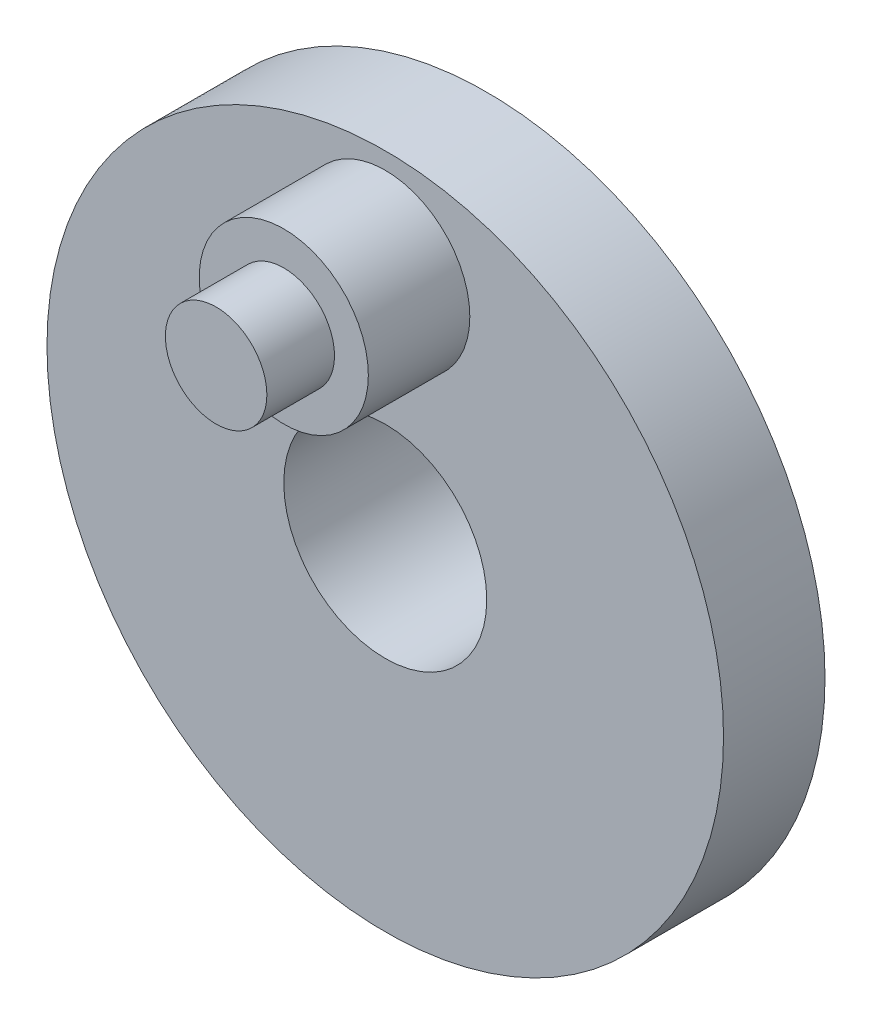
from build123d import *

# Parameters (mm, degrees)
SKETCH1_R           = 10
BOSS_EXTRUDE1_DEPTH = 3
SKETCH2_R           = 2.5
BOSS_EXTRUDE2_DEPTH = 3
SKETCH3_R           = 1.5
BOSS_EXTRUDE3_DEPTH = 2
SKETCH4_R           = 3
CUT_EXTRUDE1_DEPTH  = 24
BOSS_EXTRUDE4_START = 4
SKETCH5_R           = 4
SKETCH5_R_2         = 3
BOSS_EXTRUDE4_DEPTH = 4
SKETCH6_R           = 1
CUT_EXTRUDE2_DEPTH  = 5


with BuildPart() as part:
    # Sketch1 → Boss-Extrude1 (new body)
    with BuildSketch(Plane.XY):
        Circle(SKETCH1_R)
    extrude(amount=BOSS_EXTRUDE1_DEPTH)

    # Sketch2 → Boss-Extrude2 (add)
    with BuildSketch(Plane.XY.offset(3)):
        with Locations((0, 7)):
            Circle(SKETCH2_R)
    extrude(amount=BOSS_EXTRUDE2_DEPTH)

    # Sketch3 → Boss-Extrude3 (add)
    with BuildSketch(Plane.XY.offset(6)):
        with Locations((0, 7)):
            Circle(SKETCH3_R)
    extrude(amount=BOSS_EXTRUDE3_DEPTH)

    # Sketch4 → Cut-Extrude1 (cut)
    with BuildSketch(Plane(origin=(0, 0, 0), x_dir=(-1, 0, 0), z_dir=(0, 0, -1))):
        Circle(SKETCH4_R)
    extrude(amount=-CUT_EXTRUDE1_DEPTH, mode=Mode.SUBTRACT)

    # Sketch5 → Boss-Extrude4 (add)
    with BuildSketch(Plane(origin=(0, 0, 0), x_dir=(-1, 0, 0), z_dir=(0, 0, -1)).offset(BOSS_EXTRUDE4_START)):
        with Locations(Location((0, 0, 0), (0, 0, 180))):
            Circle(SKETCH5_R)
        Circle(SKETCH5_R_2, mode=Mode.SUBTRACT)
    extrude(amount=-BOSS_EXTRUDE4_DEPTH)

    # Sketch6 → Cut-Extrude2 (cut, symmetric)
    with BuildSketch(Plane(origin=(0, 0, 0), x_dir=(0, 0, -1), z_dir=(1, 0, 0))):
        with Locations((2, 0)):
            Circle(SKETCH6_R)
    extrude(amount=CUT_EXTRUDE2_DEPTH, both=True, mode=Mode.SUBTRACT)


solid = part.part
